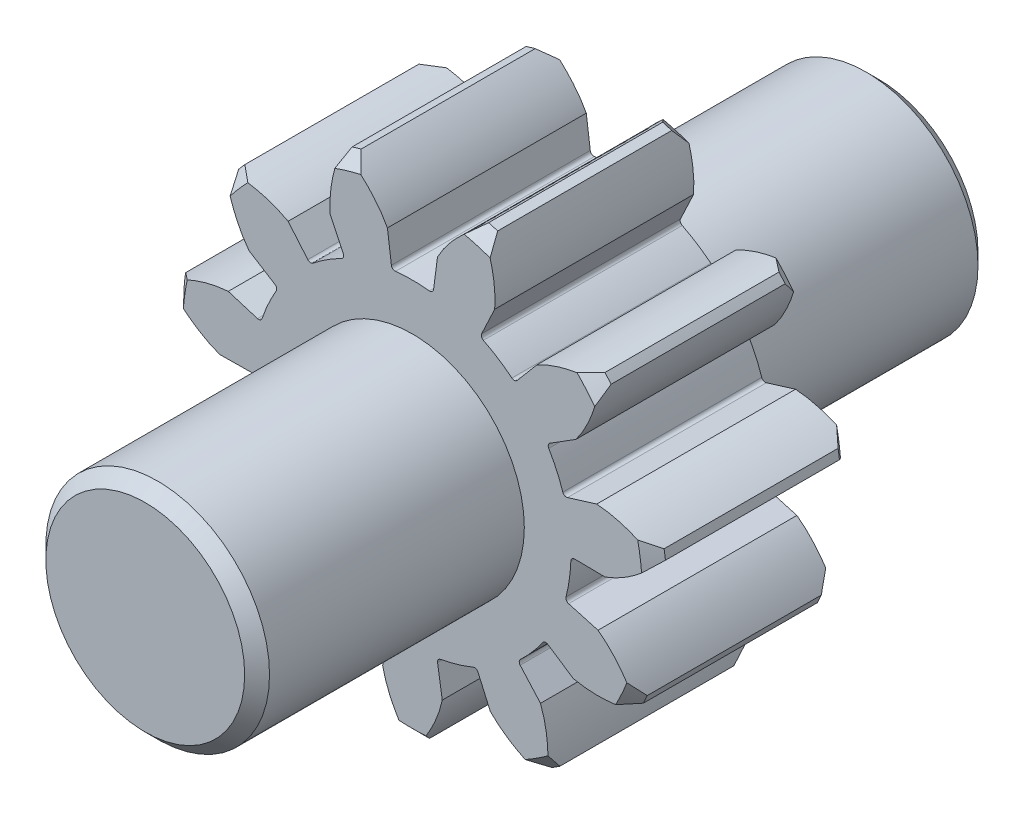
from build123d import *

# Parameters (mm, degrees)
CIRCLE_R                 = 19.5
BLANK_DEPTH              = 8
TOOTH_CHAMFER_SIZE       = 1
GEAR_SHAPING_DEPTH       = 8
FILLET2_R                = 0.3
CIRPATTERN2_COUNT        = 11
FILLET2_OF_CIRPATTERN2_R = 0.3
SKETCH2_R                = 9
BOSS_EXTRUDE1_DEPTH      = 21.5
BOSS_EXTRUDE2_START      = -59
SKETCH3_R                = 9
BOSS_EXTRUDE2_DEPTH      = 59
CHAMFER1_SIZE            = 1


with BuildPart() as part:
    # Circle → Blank (new, symmetric)
    with BuildSketch(Plane.XY):
        Circle(CIRCLE_R)
    extrude(amount=BLANK_DEPTH, both=True)

    # Tooth chamfer
    tooth_chamfer_edges = [part.edges().sort_by_distance(p)[0] for p in [
        (-19.5, 0, -8),
        (-19.5, 0, 8),
    ]]
    chamfer(tooth_chamfer_edges, length=TOOTH_CHAMFER_SIZE)

    # Tooth profile → Gear shaping (cut, symmetric)
    with BuildSketch(Plane.XY):
        with BuildLine():
            ThreePointArc((-1.657319875, 12.641827037), (0, 12.75), (1.657319875, 12.641827037))
            Line((1.657319875, 12.641827037), (2.015421626, 15.373382045))
            add(Edge.make_bspline(
                [(2.015421626, 15.373382045), (2.101128121, 15.535173288), (2.381258182, 16.022451997), (2.940334149, 16.812235008), (3.736790612, 17.674048579), (4.482655711, 18.321814632), (4.965077907, 18.691820635), (5.129920603, 18.813131441)],
                knots=[0.02088102, 0.02088102, 0.02088102, 0.02088102, 0.02088102, 0.029959916, 0.048733667, 0.068727063, 0.078876106, 0.078876106, 0.078876106, 0.078876106, 0.078876106], degree=4))
            ThreePointArc((5.129920603, 18.813131441), (0, 19.5), (-5.129920604, 18.813131441))
            add(Edge.make_bspline(
                [(-2.015421626, 15.373382045), (-2.101128121, 15.535173287), (-2.381258181, 16.022451997), (-2.940334148, 16.812235007), (-3.736790612, 17.674048577), (-4.482655711, 18.321814631), (-4.965077907, 18.691820635), (-5.129920604, 18.813131441)],
                knots=[0.02088102, 0.02088102, 0.02088102, 0.02088102, 0.02088102, 0.029959916, 0.048733667, 0.068727063, 0.078876106, 0.078876106, 0.078876106, 0.078876106, 0.078876106], degree=4))
            Line((-2.015421626, 15.373382045), (-1.657319875, 12.641827037))
        make_face()
    gear_shaping = extrude(amount=GEAR_SHAPING_DEPTH, both=True, mode=Mode.SUBTRACT)

    # Fillet2
    fillet2_edges = [part.edges().sort_by_distance(p)[0] for p in [
        (1.657319875, 12.641827037, 0),
        (-1.657319875, 12.641827037, 0),
    ]]
    fillet(fillet2_edges, radius=FILLET2_R)

    # CirPattern2: Gear shaping ×11 about axis
    cirpattern2_axis = Axis((0, 0, 8), (0, 0, -1))
    for i in range(1, CIRPATTERN2_COUNT):
        add(gear_shaping.rotate(cirpattern2_axis, i * 360 / CIRPATTERN2_COUNT), mode=Mode.SUBTRACT)

    # Fillet2 of CirPattern2
    fillet2_of_cirpattern2_edges = [part.edges().sort_by_distance(p)[0] for p in [
        (8.228913903, 9.738966885, 0),
        (5.440461504, 11.530996428, 0),
        (12.18788591, 3.744053559, 0),
        (10.810934795, 6.759155927, 0),
        (12.277290256, -3.439570318, 0),
        (12.749012676, -0.158668822, 0),
        (8.468741693, -9.531154922, 0),
        (10.639369112, -7.026117342, 0),
        (1.97142748, -12.596665181, 0),
        (5.151801029, -11.66282325, 0),
        (-5.151801029, -11.66282325, 0),
        (-1.97142748, -12.596665181, 0),
        (-10.639369112, -7.026117342, 0),
        (-8.468741693, -9.531154922, 0),
        (-12.749012676, -0.158668822, 0),
        (-12.277290256, -3.439570318, 0),
        (-10.810934795, 6.759155927, 0),
        (-12.18788591, 3.744053559, 0),
        (-5.440461504, 11.530996428, 0),
        (-8.228913903, 9.738966885, 0),
    ]]
    fillet(fillet2_of_cirpattern2_edges, radius=FILLET2_OF_CIRPATTERN2_R)

    # Sketch2 → Boss-Extrude1 (add)
    with BuildSketch(Plane.XY.offset(8)):
        Circle(SKETCH2_R)
    extrude(amount=BOSS_EXTRUDE1_DEPTH)

    # Sketch3 → Boss-Extrude2 (add)
    with BuildSketch(Plane.XY.offset(29.5).offset(BOSS_EXTRUDE2_START)):
        Circle(SKETCH3_R)
    extrude(amount=BOSS_EXTRUDE2_DEPTH)

    # Chamfer1
    chamfer1_edges = [part.edges().sort_by_distance(p)[0] for p in [
        (-9, 0, 29.5),
        (-9, 0, -29.5),
    ]]
    chamfer(chamfer1_edges, length=CHAMFER1_SIZE)


solid = part.part
